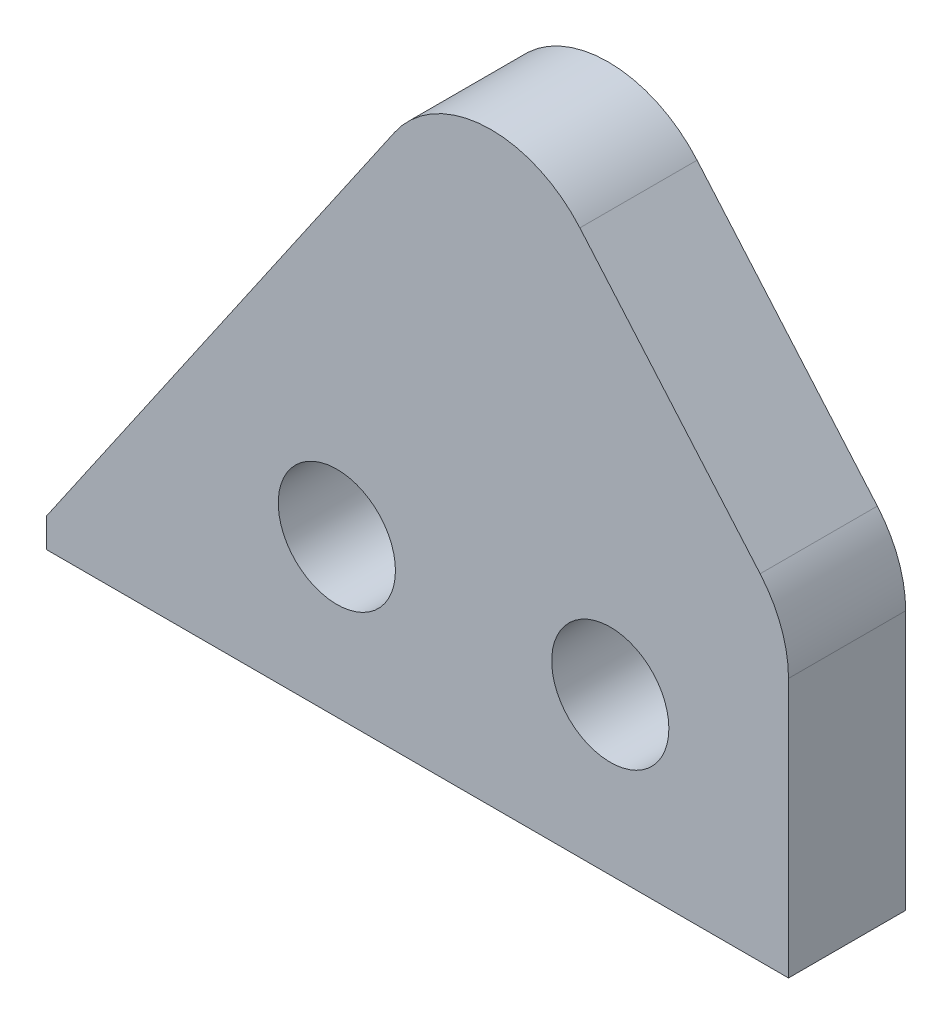
SolidWorks part; units mm, degrees
material "Q235B"
ref_plane "Front Plane" through (0, 0, 0) normal (0, 0, 1) x (1, 0, 0)
ref_plane "Top Plane" through (0, 0, 0) normal (0, 1, 0) x (1, 0, 0)
ref_plane "Right Plane" through (0, 0, 0) normal (1, 0, 0) x (0, 0, -1)
sketch "Sketch1" plane through (0, 0, 0) normal (0, 0, 1) x (1, 0, 0)
  line L0 (137442.7922, -173144.9181) -> (137353.6595, -173274.5656)
  line L1 (137543.6595, -173281.9432) -> (137543.6595, -173215.5242)
  line L2 (137536.3964, -173195.9529) -> (137490.2503, -173142.3427)
  line L3 (137353.6595, -173274.5656) -> (137353.6595, -173281.9432)
  line L4 (137353.6595, -173281.9432) -> (137543.6595, -173281.9432)
  arc A0 (137490.2503, -173142.3427) -> (137442.7922, -173144.9181) centre (137467.5134, -173161.914) ccw
  arc A1 (137543.6595, -173215.5242) -> (137536.3964, -173195.9529) centre (137513.6595, -173215.5242) ccw
  circle A2 centre (137498.0346, -173241.9432) radius 15
  circle A3 centre (137428.0346, -173241.9432) radius 15
extrude "Boss-Extrude1" add sketch "Sketch1" along normal blind 30
